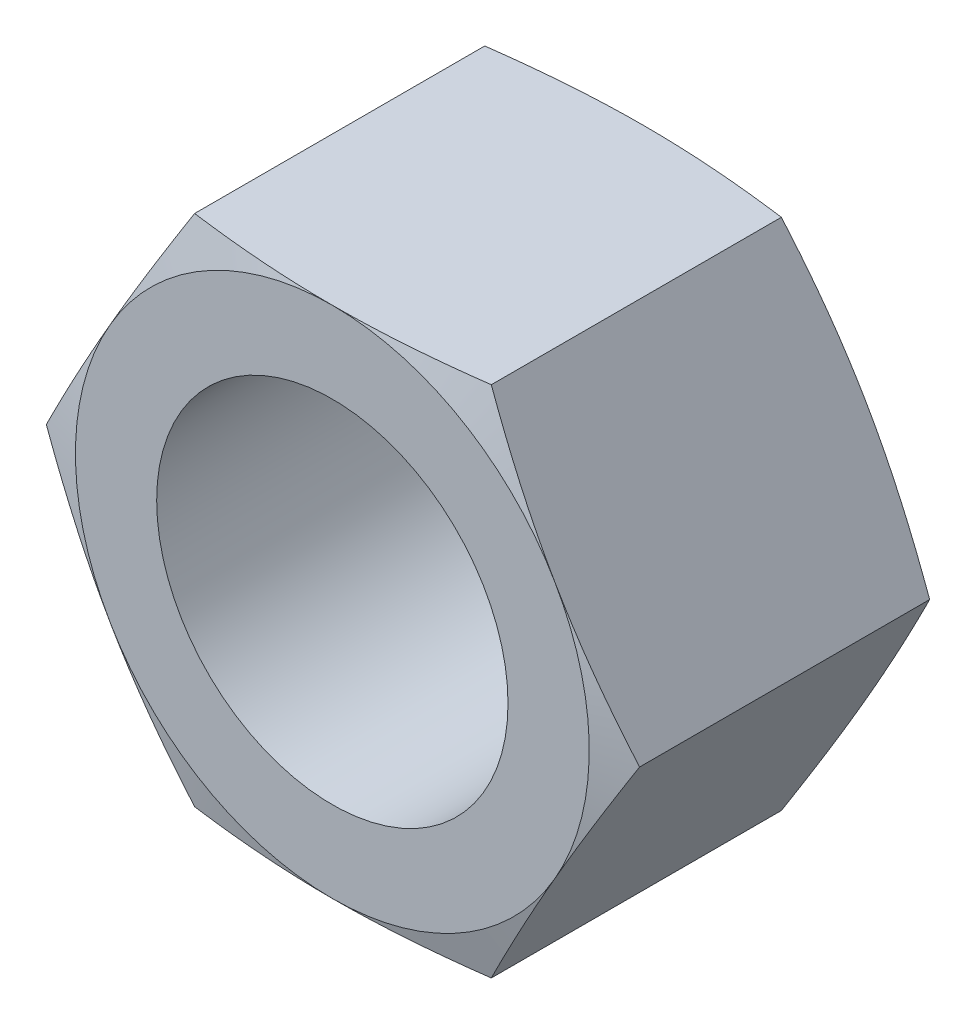
SolidWorks part; units mm, degrees
ref_plane "Plane1" through (0, 0, 0) normal (0, 0, 1) x (1, 0, 0)
ref_plane "Plane2" through (0, 0, 0) normal (0, 1, 0) x (1, 0, 0)
ref_plane "Plane3" through (0, 0, 0) normal (1, 0, 0) x (0, 0, -1)
sketch "dimension sketch" plane through (0, 0, 0) normal (0, 0, 1) x (1, 0, 0)
  line L0 (0, 0) -> (24.1005, 0)
  point P3 (36, 0)
  point P4 (1.5, 0)
  point P5 (60.79, 0)
  point P6 (31.9, 0)
  point P7 (6.4, 0)
  point P8 (55, 0)
sketch "Sketch1" plane through (0, 0, 0) normal (0, 0, 1) x (1, 0, 0)
  line L0 (-26.8088, 0) -> (37.1748, 0) construction
  line L1 (0, 25.0215) -> (0, -25.0215) construction
  line L3 (15.1975, 26.3228) -> (-15.1975, 26.3228)
  line L4 (-15.1975, 26.3228) -> (-30.395, 0)
  line L5 (-30.395, 0) -> (-15.1975, -26.3228)
  line L6 (-15.1975, -26.3228) -> (15.1975, -26.3228)
  line L7 (15.1975, -26.3228) -> (30.395, 0)
  line L8 (30.395, 0) -> (15.1975, 26.3228)
  circle A0 centre (0, 0) radius 26.3228 construction
  circle A1 centre (0, 0) radius 18
extrude "Base-Extrude" add sketch "Sketch1" along normal blind 31.9
cosmetic thread "Cosmetic Thread1" parameters "D2"=37.8
sketch "Sketch2" plane through (0, 0, 0) normal (0, 0, -1) x (-1, 0, 0)
  line L0 (-15.1975, 26.3228) -> (15.1975, 26.3228) construction
  circle A0 centre (0, 0) radius 26.3228
  circle A1 centre (0, 0) radius 18 construction
extrude "Cut-Extrude1" cut sketch "Sketch2" against normal blind 38 draft 75 flip side to cut
sketch "Sketch3" plane through (0, 0, 31.9) normal (0, 0, 1) x (1, 0, 0)
  line L0 (30.395, 0) -> (15.1975, 26.3228) construction
  circle A0 centre (0, 0) radius 26.3228
extrude "Cut-Extrude2" cut sketch "Sketch3" against normal blind 38 draft 75 flip side to cut
chamfer "Chamfer1" [suppressed] distance 0.2 angle 45
equation "\"e@Sketch1\" = \"e@dimension sketch\""
equation "\"D@Sketch1\" = \"D@dimension sketch\""
equation "\"m@Base-Extrude\" = \"m@dimension sketch\""
equation "\"D2@Cosmetic Thread1\" = 1.05 * \"D@dimension sketch\""
